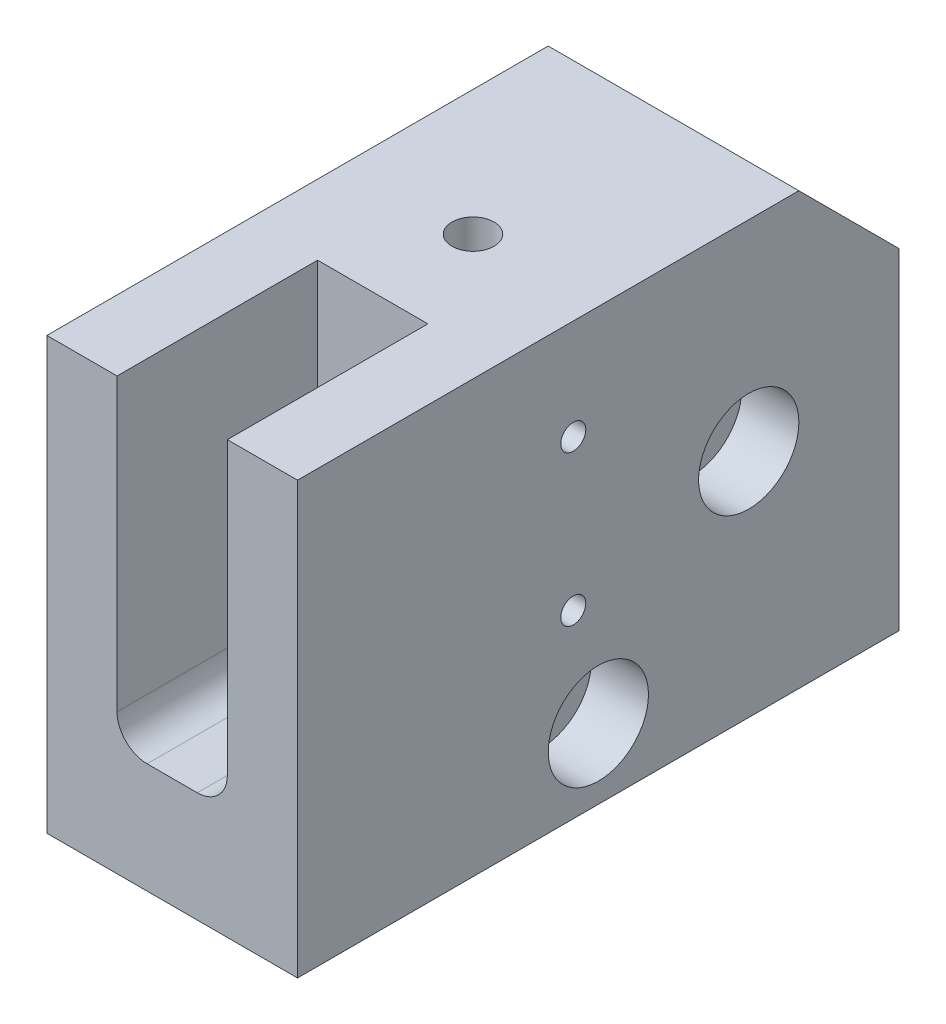
SolidWorks part; units mm, degrees
ref_plane "Front Plane" through (0, 0, 0) normal (0, 0, 1) x (1, 0, 0)
ref_plane "Top Plane" through (0, 0, 0) normal (0, 1, 0) x (1, 0, 0)
ref_plane "Right Plane" through (0, 0, 0) normal (1, 0, 0) x (0, 0, -1)
sketch "Sketch1" plane through (0, 0, 0) normal (0, 0, 1) x (1, 0, 0)
  line L0 (0, 60) -> (0, 0)
  line L1 (0, 0) -> (35, 0)
  dimension "D1" = 35
  dimension "D2" = 60
extrude "Extrude-Thin1" add sketch "Sketch1" along normal mid plane 60 thin
sketch "Sketch2" plane through (0, 0, 30) normal (0, 0, 1) x (1, 0, 0)
  line L0 (35, 0) -> (35, -25) construction
  line L1 (-25, -25) -> (35, -25)
  line L2 (-25, -25) -> (-25, -12.5)
  line L3 (-25, -12.5) -> (35, -12.5)
  line L4 (35, -25) -> (35, -12.5)
extrude "Cut-Extrude1" cut sketch "Sketch2" against normal through all
sketch "Sketch3" plane through (0, 0, 30) normal (0, 0, 1) x (1, 0, 0)
  line L0 (-12.5, 60) -> (-12.5, 16.8147) construction
  line L1 (-25, 60) -> (0, 60) construction
  line L3 (-18, 60) -> (-7, 60)
  line L4 (-18, 60) -> (-18, 28)
  line L5 (-18, 28) -> (-7, 28)
  line L6 (-7, 60) -> (-7, 28)
  line L7 (-18, 60) -> (-7, 28) construction
  line L8 (-18, 28) -> (-7, 60) construction
  point P4 (-12.5, 44)
  dimension "D1" = 11
  dimension "D2" = 32
extrude "Cut-Extrude2" cut sketch "Sketch3" against normal blind 20
fillet "Fillet1" radius 3 2 edges at (-7, 28, 20) (-18, 28, 20)
sketch "Sketch6" plane through (0, 0, 10) normal (0, 0, 1) x (1, 0, 0)
  line L0 (-12.5, 60) -> (-12.5, 32.3038) construction
  line L1 (-7, 60) -> (-18, 60) construction
  circle A0 centre (-12.5, 50) radius 3
  circle A1 centre (-12.5, 35) radius 3
  dimension "D1" = 6
  dimension "D2" = 10
  dimension "D3" = 15
extrude "Cut-Extrude3" cut sketch "Sketch6" against normal blind 15
hole_wizard "M3 Tapped Hole2" positions "Sketch8" profile "Sketch7" tap size "M3" standard "GB"
sketch "Sketch8" plane through (0, 0, 0) normal (1, 0, 0) x (0, 0, -1)
  line L0 (-30, 60) -> (30, 60) construction
  line L1 (-30, 60) -> (-30, 0) construction
  point P1 (-2.5, 50)
  point P3 (-2.5, 35)
  dimension "D1" = 10
  dimension "D2" = 15
  dimension "D3" = 27.5
sketch "Sketch7" plane through (0, 50, 2.5) normal (0, 1, 0) x (0, 0, -1)
  line L0 (0, 0) -> (0, 12.2511)
  line L1 (0, 12.2511) -> (1.25, 11.5)
  line L2 (1.25, 11.5) -> (1.25, 0)
  line L5 (1.25, 0) -> (0, 0)
  line L10 (0, 12.2511) -> (-1.25, 11.5) construction
  line L11 (0, -6.35) -> (0, 107.95) construction
  dimension "螺纹孔钻头直径" = 2.5
  dimension "螺纹孔钻头深度" = 11.5
  dimension "导头角度" = 118
cosmetic thread "Cosmetic Thread5" parameters "D1"=10, "D2"=3
cosmetic thread "Cosmetic Thread6" parameters "D1"=10, "D2"=3
hole_wizard "M5 Tapped Hole1" positions "Sketch10" profile "Sketch9" tap size "M5" standard "GB"
sketch "Sketch10" plane through (0, 60, 0) normal (0, 1, 0) x (-1, 0, 0)
  line L1 (25, -30) -> (0, -30) construction
  line L2 (12.5, -30) -> (12.5, 5.1258) construction
  point P0 (12.5, 0)
  dimension "D2" = 30
sketch "Sketch9" plane through (-12.5, 60, 0) normal (1, 0, 0) x (0, 0, 1)
  line L0 (0, 0) -> (0, 13.6618)
  line L1 (0, 13.6618) -> (2.1, 12.4)
  line L2 (2.1, 12.4) -> (2.1, 0)
  line L5 (2.1, 0) -> (0, 0)
  line L10 (0, 13.6618) -> (-2.1, 12.4) construction
  line L11 (0, -6.35) -> (0, 107.95) construction
  dimension "螺纹孔钻头直径" = 4.2
  dimension "螺纹孔钻头深度" = 12.4
  dimension "导头角度" = 118
cosmetic thread "Cosmetic Thread9" parameters "D1"=10, "D2"=5
sketch "Sketch11" plane through (0, -12.5, 0) normal (0, -1, 0) x (1, 0, 0)
  line L0 (30, -5) -> (30, -25) construction
  line L1 (32.25, -5) -> (32.25, -25)
  line L2 (27.75, -5) -> (27.75, -25)
  line L3 (35, -30) -> (35, 30) construction
  line L4 (35, -30) -> (-25, -30) construction
  arc A0 (32.25, -5) -> (27.75, -5) centre (30, -5) ccw
  arc A1 (27.75, -25) -> (32.25, -25) centre (30, -25) ccw
  point P2 (30, -15)
  dimension "D1" = 4.5
  dimension "D2" = 5
  dimension "D3" = 20
  dimension "D4" = 5
extrude "Cut-Extrude4" cut sketch "Sketch11" against normal through all
sketch "Sketch12" plane through (0, 0, 30) normal (0, 0, 1) x (1, 0, 0)
  line L0 (35, -12.5) -> (-25, -12.5) construction
  line L1 (-12.5, 60) -> (-12.5, -15.6366) construction
  line L2 (-7, 60) -> (-18, 60) construction
  circle A0 centre (-12.5, 17.5) radius 5
  circle A1 centre (-12.5, 2.5) radius 5
  dimension "D1" = 10
  dimension "D2" = 15
  dimension "D3" = 15
extrude "Cut-Extrude5" [suppressed] cut sketch "Sketch12" against normal through all
sketch "Sketch13" plane through (0, 0, 30) normal (0, 0, 1) x (1, 0, 0)
  line L1 (35, -12.5) -> (0, -12.5)
  line L2 (35, -12.5) -> (35, 0)
  line L3 (35, 0) -> (0, 0)
  line L4 (0, -12.5) -> (0, 0)
extrude "Cut-Extrude6" cut sketch "Sketch13" against normal blind 1
sketch "Sketch14" plane through (0, 0, 0) normal (0, 1, 0) x (1, 0, 0)
  line L0 (35, -29) -> (0, -29) construction
  line L1 (35, 30) -> (25, 30)
  line L2 (35, 30) -> (35, -29)
  line L3 (35, -29) -> (25, -29)
  line L4 (25, 30) -> (25, -29)
  dimension "D1" = 10
extrude "Cut-Extrude7" cut sketch "Sketch14" against normal blind 1.5
chamfer "Chamfer1" distance 10 angle 45 1 edges at (-12.5, 60, -30)
sketch "Sketch15" plane through (0, 0, 29) normal (0, 0, 1) x (1, 0, 0)
  line L1 (0, 0) -> (35, 0)
  line L2 (0, 0) -> (0, -12.5)
  line L3 (0, -12.5) -> (35, -12.5)
  line L4 (35, 0) -> (35, -12.5)
extrude "Cut-Extrude8" cut sketch "Sketch15" against normal through all
hole_wizard "Hole Size per Socket Head Cap Screw Type1" positions "Sketch17" profile "Sketch16" counterbore size "M5" standard "GB" end condition through all
sketch "Sketch17" plane through (0, 0, 0) normal (1, 0, 0) x (0, 0, -1)
  line L3 (-30, 60) -> (20, 60) construction
  line L4 (30, 50) -> (30, -12.5) construction
  point P0 (0, 24)
  point P1 (15, 40)
  dimension "D1" = 36
  dimension "D2" = 20
  dimension "D3" = 15
  dimension "D4" = 30
sketch "Sketch16" plane through (0, 24, 0) normal (0, 1, 0) x (0, 0, -1)
  line L0 (0, 0) -> (0, 25)
  line L1 (0, 25) -> (2.75, 25)
  line L3 (2.75, 25) -> (2.75, 5.7)
  line L4 (2.75, 5.7) -> (5, 5.7)
  line L5 (5, 5.7) -> (5, 0)
  line L7 (5, 0) -> (0, 0)
  line L11 (0, -6.35) -> (0, 107.95) construction
  dimension "通孔孔直径" = 5.5
  dimension "通孔孔深度" = 25
  dimension "柱形沉头孔直径" = 10
  dimension "柱形沉头孔深度" = 5.7
sketch "Sketch18" plane through (-25, 0, 0) normal (-1, 0, 0) x (0, 0, 1)
  line L0 (-30, 50) -> (-30, -12.5) construction
  line L1 (30, -12.5) -> (-30, -12.5)
  line L2 (30, -12.5) -> (30, 17)
  line L3 (30, 17) -> (-30, 17)
  line L4 (-30, -12.5) -> (-30, 17)
  dimension "D1" = 17
extrude "Cut-Extrude9" cut sketch "Sketch18" against normal through all
sketch "Sketch19" plane through (-25, 0, 0) normal (-1, 0, 0) x (0, 0, 1)
  circle A0 centre (-15, 40) radius 5
  circle A1 centre (0, 24) radius 5
  dimension "D1" = 10
extrude "Cut-Extrude10" cut sketch "Sketch19" against normal blind 5.7
